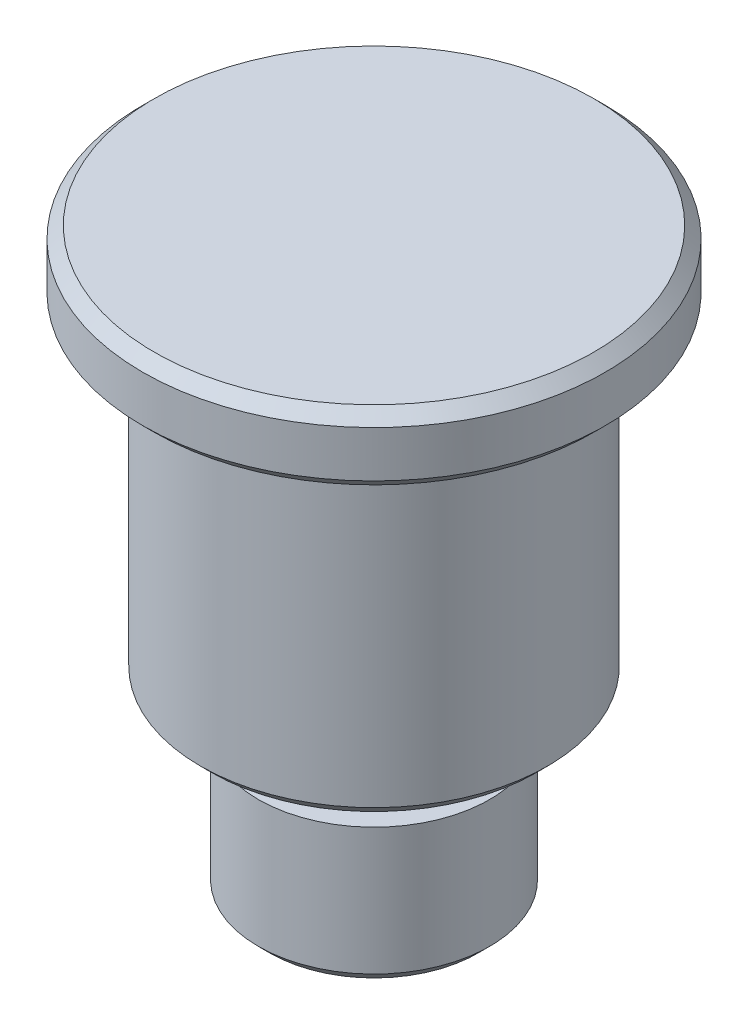
SolidWorks part; units mm, degrees
material "45#"
ref_plane "Front Plane" through (0, 0, 0) normal (0, 0, 1) x (1, 0, 0)
ref_plane "Top Plane" through (0, 0, 0) normal (0, 1, 0) x (1, 0, 0)
ref_plane "Right Plane" through (0, 0, 0) normal (1, 0, 0) x (0, 0, -1)
sketch "Sketch1" plane through (0, 0, 0) normal (1, 0, 0) x (0, 0, -1)
  line L0 (0, 0) -> (0, -41.4307) construction
  line L1 (0, 0) -> (10, 0)
  line L2 (10, 0) -> (10, -3)
  line L3 (10, -3) -> (7.5, -3)
  line L4 (7.5, -3) -> (7.5, -17)
  line L5 (7.5, -17) -> (4, -17)
  line L6 (4, -17) -> (4, -19)
  line L7 (4, -19) -> (5, -19)
  line L8 (5, -19) -> (5, -25)
  line L9 (5, -25) -> (0, -25)
  line L10 (0, 0) -> (0, -25)
  dimension "D1" = 15
  dimension "D2" = 10
  dimension "D3" = 1
  dimension "D4" = 2
  dimension "D5" = 14
  dimension "D6" = 3
  dimension "D7" = 20
  dimension "D8" = 8
revolve "Revolve1" add sketch "Sketch1" angle 360 about L0
cosmetic thread "Cosmetic Thread1" parameters "D2"=8.376
chamfer "Chamfer1" distance 0.5 angle 45 4 edges at (0, 0, 10) (0, -3, 10) (0, -17, 7.5) (0, -25, 5)
